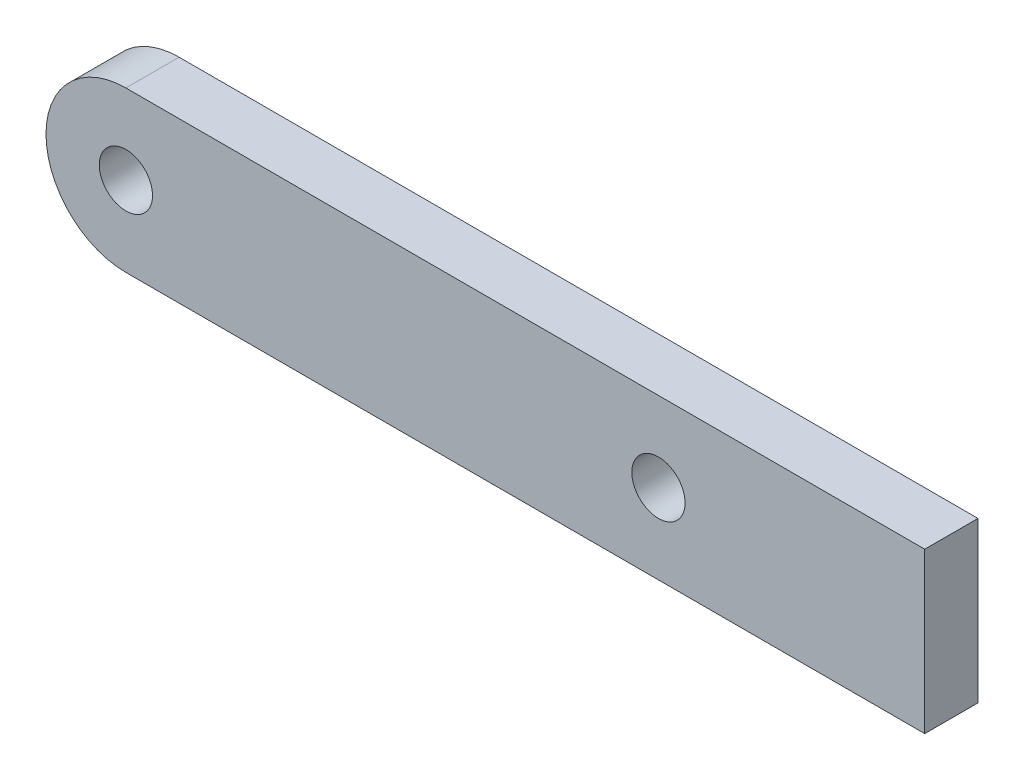
SolidWorks part; units mm, degrees
ref_plane "Front Plane" through (0, 0, 0) normal (0, 0, 1) x (1, 0, 0)
ref_plane "Top Plane" through (0, 0, 0) normal (0, 1, 0) x (1, 0, 0)
ref_plane "Right Plane" through (0, 0, 0) normal (1, 0, 0) x (0, 0, -1)
sketch "Sketch1" plane through (0, 0, 0) normal (0, 0, 1) x (1, 0, 0)
  line L0 (0, 150) -> (1500, 150)
  line L1 (1500, 150) -> (1500, -150)
  line L2 (1500, -150) -> (0, -150)
  arc A0 (0, 150) -> (0, -150) centre (0, 0) ccw
  circle A1 centre (1000, 0) radius 50
  circle A2 centre (0, 0) radius 50
  dimension "D1" = 300
  dimension "D2" = 100
  dimension "D3" = 100
  dimension "D4" = 1000
  dimension "D5" = 1500
extrude "Boss-Extrude1" add sketch "Sketch1" along normal blind 100
